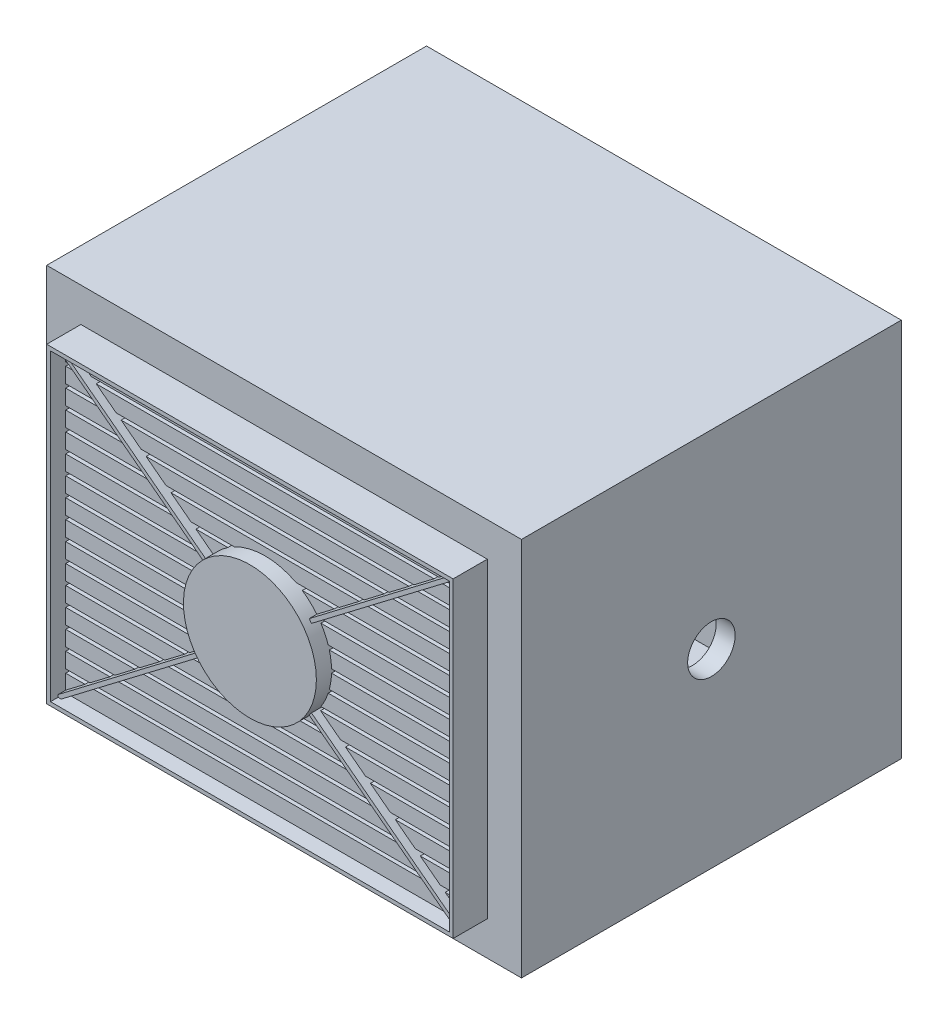
SolidWorks part; units mm, degrees
ref_plane "Front Plane" through (0, 0, 0) normal (0, 0, 1) x (1, 0, 0)
ref_plane "Top Plane" through (0, 0, 0) normal (0, 1, 0) x (1, 0, 0)
ref_plane "Right Plane" through (0, 0, 0) normal (1, 0, 0) x (0, 0, -1)
sketch "Sketch1" plane through (0, 0, 0) normal (1, 0, 0) x (0, 0, -1)
  line L1 (100, 100) -> (-100, 100)
  line L2 (100, 100) -> (100, -100)
  line L3 (100, -100) -> (-100, -100)
  line L4 (-100, 100) -> (-100, -100)
  line L5 (100, 100) -> (-100, -100) construction
  line L6 (100, -100) -> (-100, 100) construction
  point P0 (0, 0)
  dimension "D1" = 200
  dimension "D2" = 200
extrude "Boss-Extrude1" add sketch "Sketch1" along normal mid plane 250
sketch "Sketch2" plane through (0, 0, 100) normal (0, 0, 1) x (1, 0, 0)
  line L0 (125, 100) -> (125, -100) construction
  line L1 (-105, 80) -> (105, 80)
  line L2 (-105, 80) -> (-105, -80)
  line L3 (-105, -80) -> (105, -80)
  line L4 (105, 80) -> (105, -80)
  line L5 (-105, 80) -> (105, -80) construction
  line L6 (-105, -80) -> (105, 80) construction
  line L7 (125, 100) -> (-125, 100) construction
  point P0 (0, 0)
  dimension "D1" = 20
  dimension "D2" = 20
extrude "Boss-Extrude2" add sketch "Sketch2" along normal blind 10
sketch "Sketch8" plane through (0, 0, 110) normal (0, 0, 1) x (1, 0, 0)
  line L0 (-105, 0) -> (105, 0)
  line L1 (-105, 80) -> (-105, -80) construction
  line L2 (105, -80) -> (105, 80) construction
extrude "Cut-Extrude-Thin5" cut sketch "Sketch8" against normal blind 2 thin thin type mid plane wall 2
pattern_linear "LPattern1" count 8 spacing 10 along (0, 1, 0) count 8 spacing 10 along (0, -1, 0) seed only of "Cut-Extrude-Thin5"
sketch "Sketch11" plane through (0, 0, 100) normal (0, 0, 1) x (1, 0, 0)
  circle A0 centre (0, 0) radius 35
  dimension "D1" = 70
extrude "Boss-Extrude9" add sketch "Sketch11" along normal blind 18
sketch "Sketch12" plane through (0, 0, 100) normal (0, 0, 1) x (1, 0, 0)
  line L0 (-105, 80) -> (105, -80)
extrude "Extrude-Thin2" add sketch "Sketch12" along normal blind 14 thin thin type mid plane wall 2
sketch "Sketch13" plane through (0, 0, 100) normal (0, 0, 1) x (1, 0, 0)
  line L0 (105, 80) -> (-105, -80)
  line L1 (-105, -80) -> (103.35, -80) construction
  line L2 (-105, -71) -> (-105, -80) construction
extrude "Extrude-Thin3" add sketch "Sketch13" along normal blind 14 thin thin type mid plane wall 2
sketch "Sketch14" plane through (0, 0, 100) normal (0, 0, 1) x (1, 0, 0)
  line L0 (104.394, 80.7954) -> (105.606, 79.2046) construction
  line L1 (-105, -80) -> (105, -80)
  line L2 (-105, -80) -> (-105, 80)
  line L3 (-105, 80) -> (105, 80)
  line L4 (105, -80) -> (105, 80)
  line L5 (-105, -80) -> (105, 80) construction
  line L6 (-105, 80) -> (105, -80) construction
  line L7 (-107, 82) -> (107, 82)
  line L8 (107, -82) -> (107, 82)
  line L9 (-107, -82) -> (107, -82)
  line L10 (-107, -82) -> (-107, 82)
  point P0 (0, 0)
  dimension "D1" = 2
extrude "Boss-Extrude10" add sketch "Sketch14" along normal up to surface (18 mm away) up to face at (35, 0, 118)
sketch "Sketch15" plane through (-125, 0, 0) normal (-1, 0, 0) x (0, 0, 1)
  line L8 (90, -90) -> (90, 90)
  line L9 (90, 90) -> (-90, 90)
  line L10 (-90, 90) -> (-90, -90)
  line L11 (-90, -90) -> (90, -90)
  line L12 (90, -90) -> (90, 90)
  line L13 (90, 90) -> (-90, 90)
  line L14 (-90, 90) -> (-90, -90)
  line L15 (-90, -90) -> (90, -90)
  dimension "D1" = 10
extrude "Cut-Extrude1" cut sketch "Sketch15" against normal offset from surface (230 mm away) 10 from offset 10 up to face at (125, 0, 0) offset against normal yes
sketch "Sketch16" plane through (125, 0, 0) normal (1, 0, 0) x (0, 0, -1)
  circle A0 centre (0, 0) radius 12.5 construction
  circle A1 centre (0, 0) radius 12.5
extrude "Cut-Extrude2" cut sketch "Sketch16" against normal blind 83
